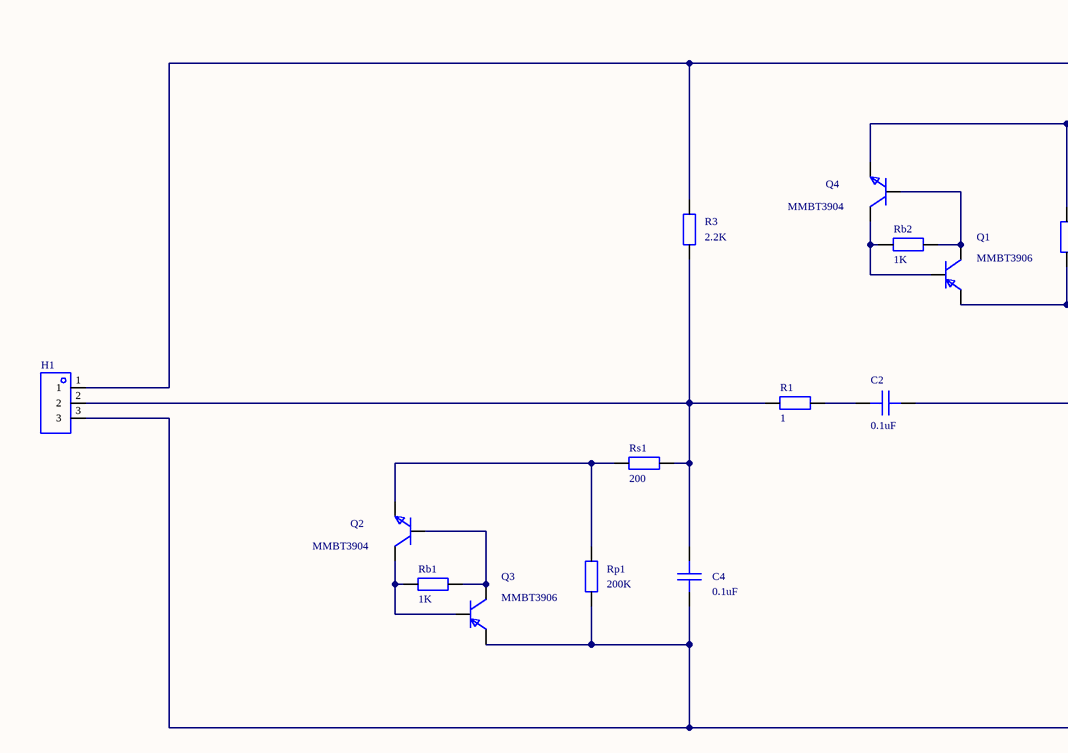
[diagram p0: MISC51432-3.schdoc, column 1 of 4]
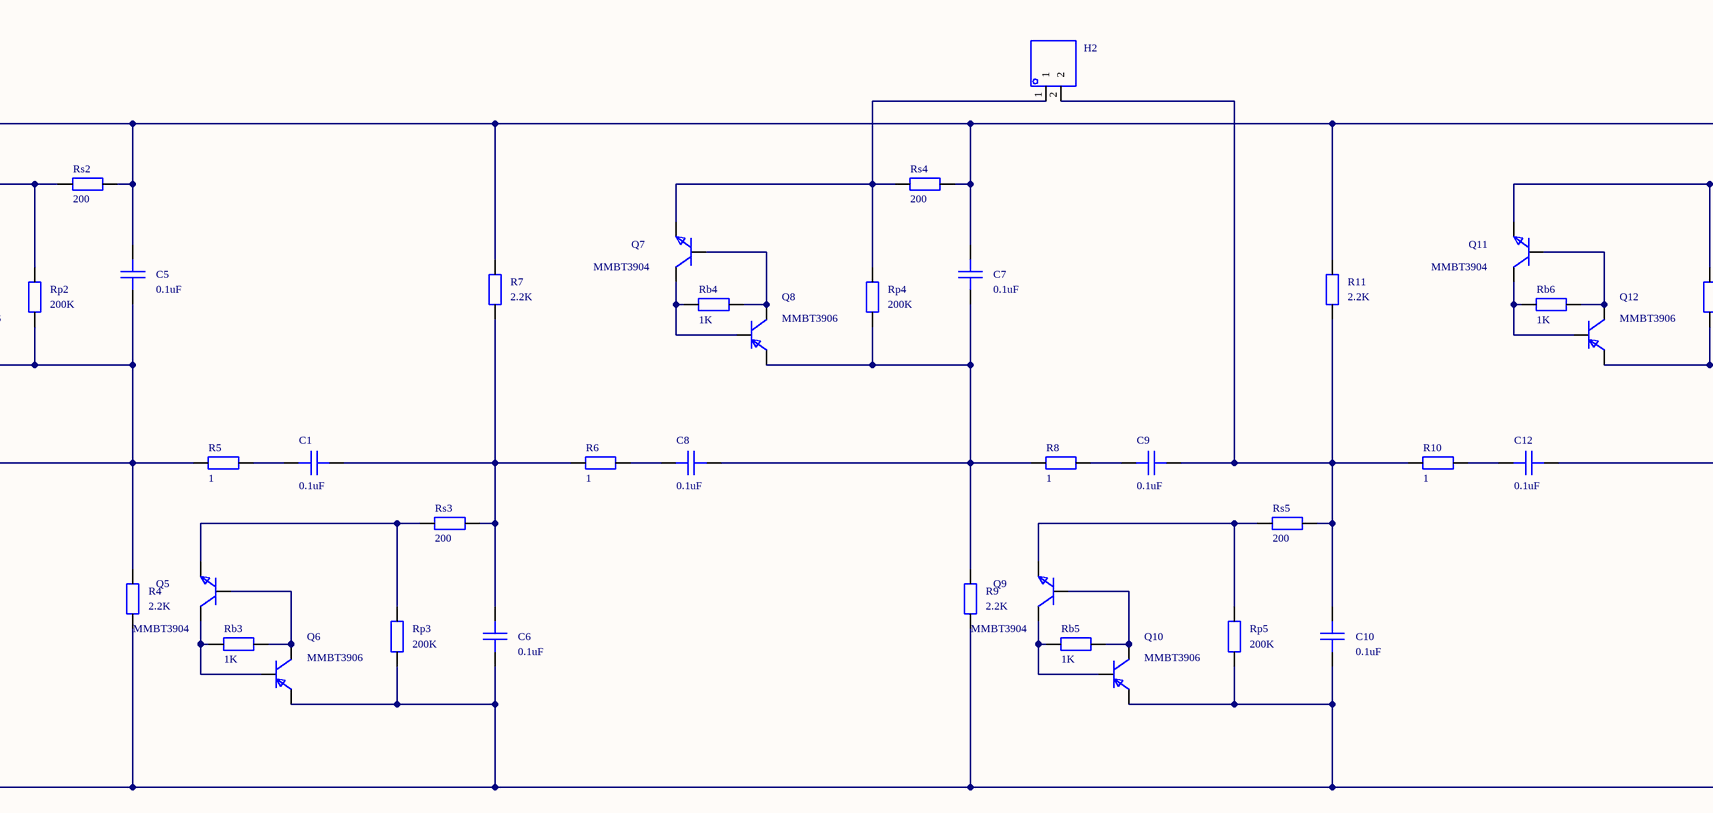
[diagram p1: MISC51432-3.schdoc, column 2 of 4]
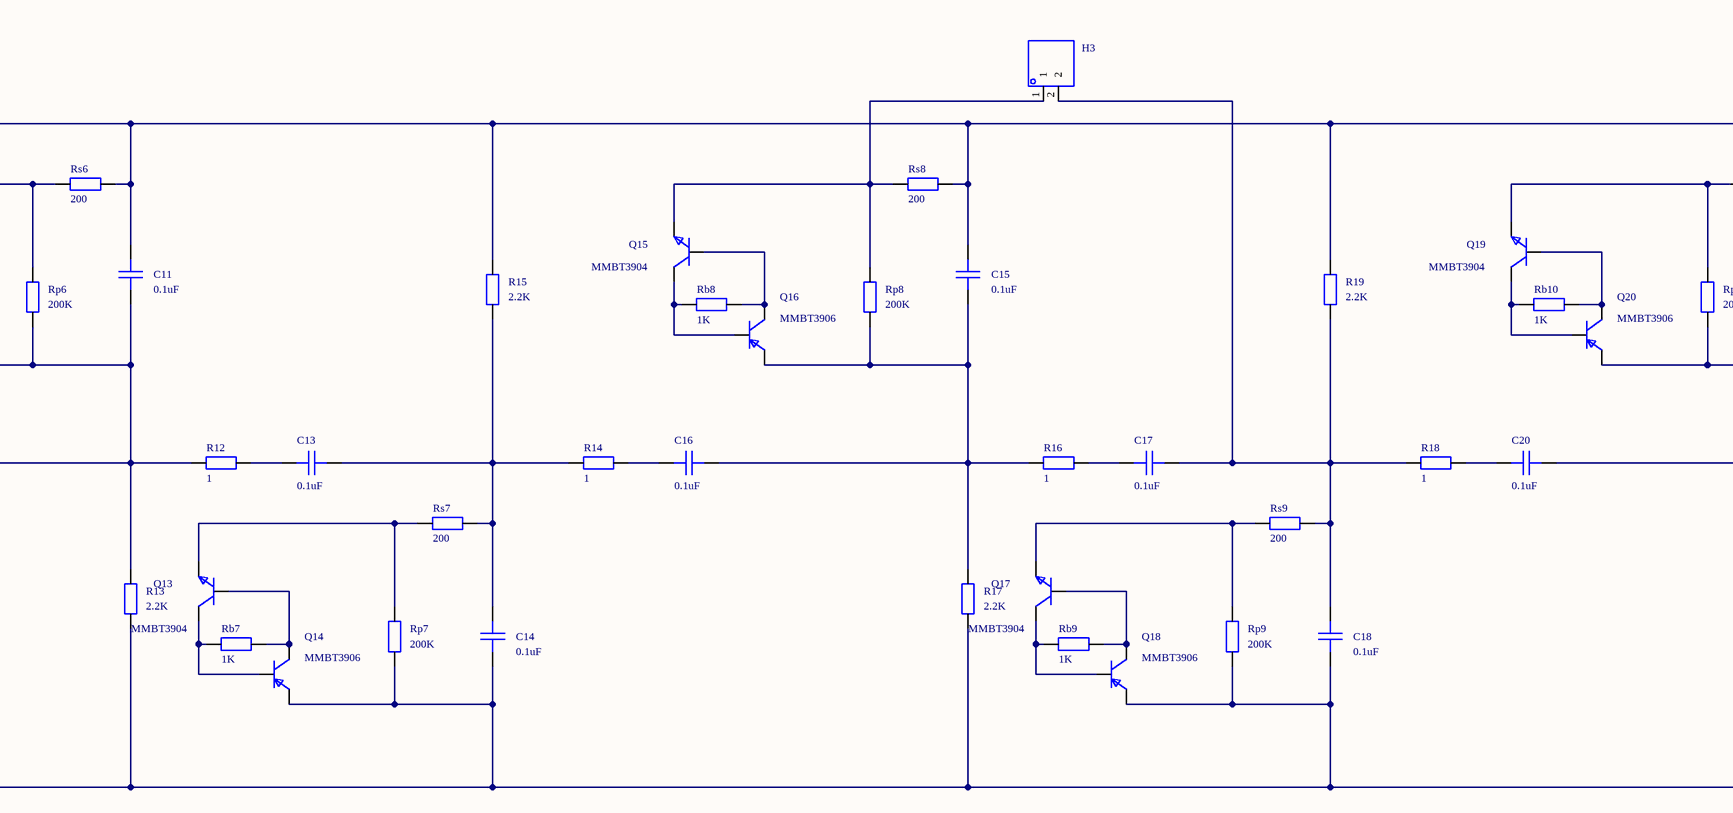
[diagram p2: MISC51432-3.schdoc, column 3 of 4]
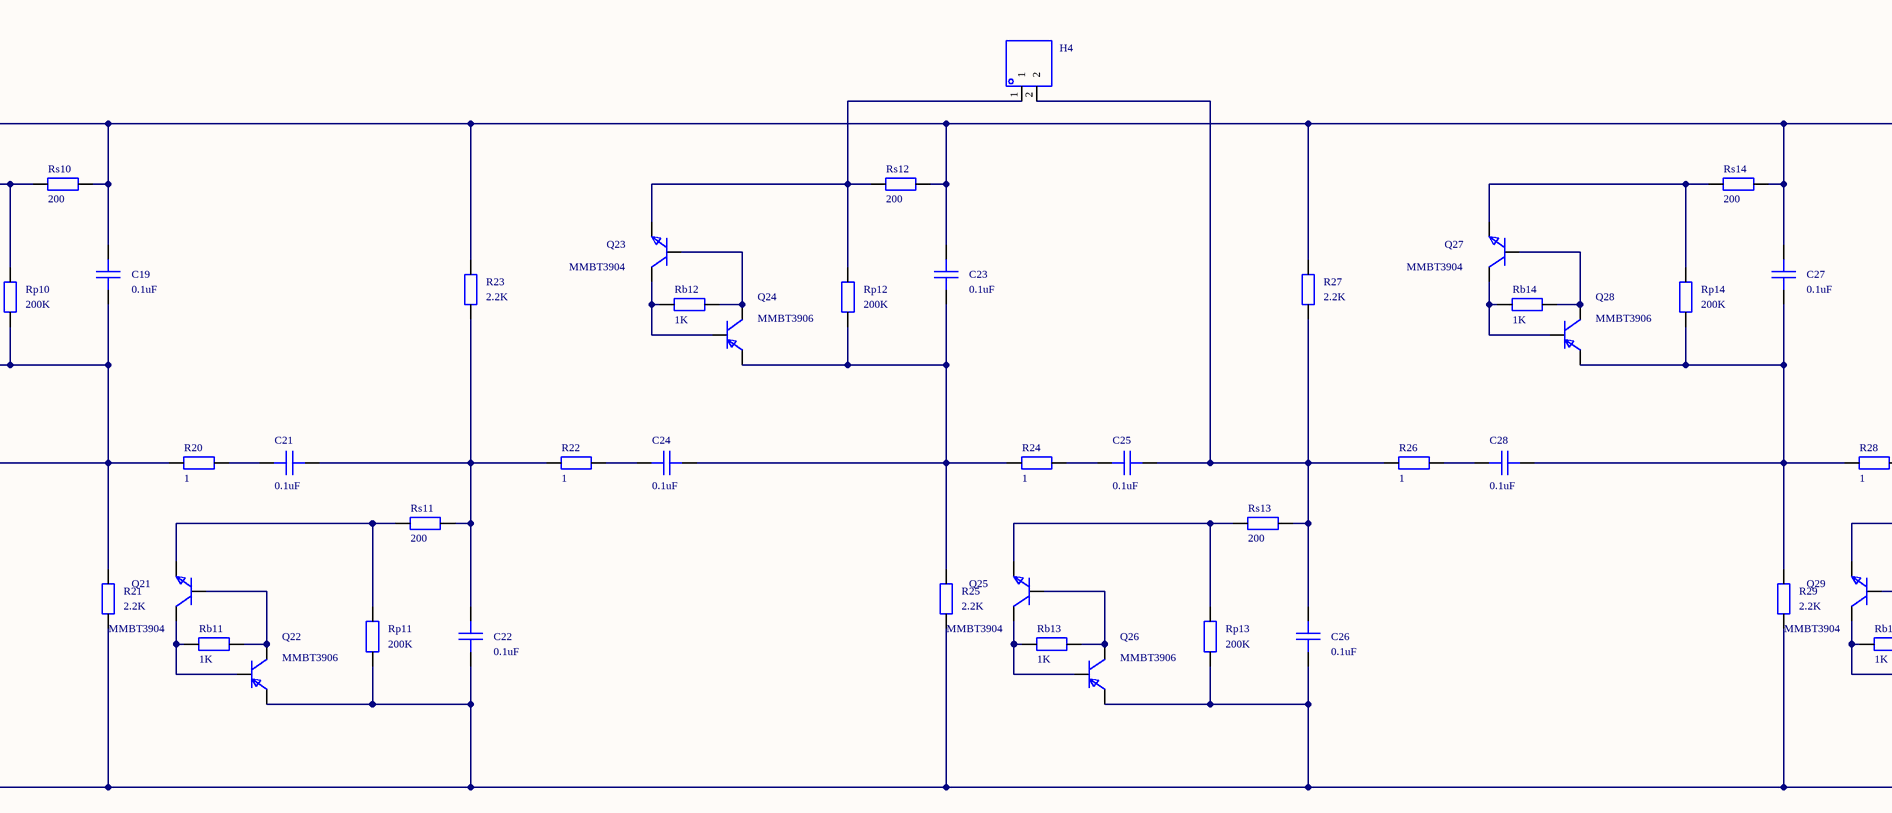
[diagram p3: MISC51432-3.schdoc, column 4 of 4]
# Altium project MISC51432-2.PrjPcb
1 sheet, 257 parts. Net scope: global (net labels, ports and power ports of the same name join across sheets).
Board file: MISC51432.pcbdoc

## Sheet MISC51432-3.schdoc
size 297 x 209 mm; Version: V1.0; @Project Name: MISC51432; @Page Count: 1; @Update Date: 2025-01-08; @Create Date: 2025-01-08; @Schematic Name: MISC51432; @Page No: 1; @Board Name: MISC51432; @Create Time: 14:24:57; @Update Time: 14:24:57

### Parts
C1  0.1uF  [C0402]
C2  0.1uF  [C0402]
C4  0.1uF  [C0402]
C5  0.1uF  [C0402]
C6  0.1uF  [C0402]
C7  0.1uF  [C0402]
C8  0.1uF  [C0402]
C9  0.1uF  [C0402]
C10  0.1uF  [C0402]
C11  0.1uF  [C0402]
C12  0.1uF  [C0402]
C13  0.1uF  [C0402]
C14  0.1uF  [C0402]
C15  0.1uF  [C0402]
C16  0.1uF  [C0402]
C17  0.1uF  [C0402]
C18  0.1uF  [C0402]
C19  0.1uF  [C0402]
C20  0.1uF  [C0402]
C21  0.1uF  [C0402]
C22  0.1uF  [C0402]
C23  0.1uF  [C0402]
C24  0.1uF  [C0402]
C25  0.1uF  [C0402]
C26  0.1uF  [C0402]
C27  0.1uF  [C0402]
C28  0.1uF  [C0402]
C29  0.1uF  [C0402]
C30  0.1uF  [C0402]
C31  0.1uF  [C0402]
C32  0.1uF  [C0402]
C33  0.1uF  [C0402]
C34  0.1uF  [C0402]
C35  0.1uF  [C0402]
C36  0.1uF  [C0402]
C37  0.1uF  [C0402]
C38  0.1uF  [C0402]
C39  0.1uF  [C0402]
C40  0.1uF  [C0402]
C41  0.1uF  [C0402]
C42  0.1uF  [C0402]
C43  0.1uF  [C0402]
C44  0.1uF  [C0402]
C45  0.1uF  [C0402]
C46  0.1uF  [C0402]
C47  0.1uF  [C0402]
C48  0.1uF  [C0402]
C49  0.1uF  [C0402]
C50  0.1uF  [C0402]
C51  0.1uF  [C0402]
C52  0.1uF  [C0402]
C53  0.1uF  [C0402]
C54  0.1uF  [C0402]
C55  0.1uF  [C0402]
C56  0.1uF  [C0402]
H1  (no value)  [HDR-TH_3P-P2.54-V-M]
H2  (no value)  [HDR-TH_2P-P2.54-V-M-1]
H3  (no value)  [HDR-TH_2P-P2.54-V-M-1]
H4  (no value)  [HDR-TH_2P-P2.54-V-M-1]
H5  (no value)  [HDR-TH_2P-P2.54-V-M-1]
H6  (no value)  [HDR-TH_2P-P2.54-V-M-1]
H7  (no value)  [HDR-TH_2P-P2.54-V-M-1]
Q1  MMBT3906  [SOT-23-3_L2.9-W1.3-P1.90-LS2.4-BR]
Q2  MMBT3904  [SOT-23-3_L2.9-W1.3-P1.90-LS2.4-BR]
Q3  MMBT3906  [SOT-23-3_L2.9-W1.3-P1.90-LS2.4-BR]
Q4  MMBT3904  [SOT-23-3_L2.9-W1.3-P1.90-LS2.4-BR]
Q5  MMBT3904  [SOT-23-3_L2.9-W1.3-P1.90-LS2.4-BR]
Q6  MMBT3906  [SOT-23-3_L2.9-W1.3-P1.90-LS2.4-BR]
Q7  MMBT3904  [SOT-23-3_L2.9-W1.3-P1.90-LS2.4-BR]
Q8  MMBT3906  [SOT-23-3_L2.9-W1.3-P1.90-LS2.4-BR]
Q9  MMBT3904  [SOT-23-3_L2.9-W1.3-P1.90-LS2.4-BR]
Q10  MMBT3906  [SOT-23-3_L2.9-W1.3-P1.90-LS2.4-BR]
Q11  MMBT3904  [SOT-23-3_L2.9-W1.3-P1.90-LS2.4-BR]
Q12  MMBT3906  [SOT-23-3_L2.9-W1.3-P1.90-LS2.4-BR]
Q13  MMBT3904  [SOT-23-3_L2.9-W1.3-P1.90-LS2.4-BR]
Q14  MMBT3906  [SOT-23-3_L2.9-W1.3-P1.90-LS2.4-BR]
Q15  MMBT3904  [SOT-23-3_L2.9-W1.3-P1.90-LS2.4-BR]
Q16  MMBT3906  [SOT-23-3_L2.9-W1.3-P1.90-LS2.4-BR]
Q17  MMBT3904  [SOT-23-3_L2.9-W1.3-P1.90-LS2.4-BR]
Q18  MMBT3906  [SOT-23-3_L2.9-W1.3-P1.90-LS2.4-BR]
Q19  MMBT3904  [SOT-23-3_L2.9-W1.3-P1.90-LS2.4-BR]
Q20  MMBT3906  [SOT-23-3_L2.9-W1.3-P1.90-LS2.4-BR]
Q21  MMBT3904  [SOT-23-3_L2.9-W1.3-P1.90-LS2.4-BR]
Q22  MMBT3906  [SOT-23-3_L2.9-W1.3-P1.90-LS2.4-BR]
Q23  MMBT3904  [SOT-23-3_L2.9-W1.3-P1.90-LS2.4-BR]
Q24  MMBT3906  [SOT-23-3_L2.9-W1.3-P1.90-LS2.4-BR]
Q25  MMBT3904  [SOT-23-3_L2.9-W1.3-P1.90-LS2.4-BR]
Q26  MMBT3906  [SOT-23-3_L2.9-W1.3-P1.90-LS2.4-BR]
Q27  MMBT3904  [SOT-23-3_L2.9-W1.3-P1.90-LS2.4-BR]
Q28  MMBT3906  [SOT-23-3_L2.9-W1.3-P1.90-LS2.4-BR]
Q29  MMBT3904  [SOT-23-3_L2.9-W1.3-P1.90-LS2.4-BR]
Q30  MMBT3906  [SOT-23-3_L2.9-W1.3-P1.90-LS2.4-BR]
Q31  MMBT3904  [SOT-23-3_L2.9-W1.3-P1.90-LS2.4-BR]
Q32  MMBT3906  [SOT-23-3_L2.9-W1.3-P1.90-LS2.4-BR]
Q33  MMBT3904  [SOT-23-3_L2.9-W1.3-P1.90-LS2.4-BR]
Q34  MMBT3906  [SOT-23-3_L2.9-W1.3-P1.90-LS2.4-BR]
Q35  MMBT3904  [SOT-23-3_L2.9-W1.3-P1.90-LS2.4-BR]
Q36  MMBT3906  [SOT-23-3_L2.9-W1.3-P1.90-LS2.4-BR]
Q37  MMBT3904  [SOT-23-3_L2.9-W1.3-P1.90-LS2.4-BR]
Q38  MMBT3906  [SOT-23-3_L2.9-W1.3-P1.90-LS2.4-BR]
Q39  MMBT3904  [SOT-23-3_L2.9-W1.3-P1.90-LS2.4-BR]
Q40  MMBT3906  [SOT-23-3_L2.9-W1.3-P1.90-LS2.4-BR]
Q41  MMBT3904  [SOT-23-3_L2.9-W1.3-P1.90-LS2.4-BR]
Q42  MMBT3906  [SOT-23-3_L2.9-W1.3-P1.90-LS2.4-BR]
Q43  MMBT3904  [SOT-23-3_L2.9-W1.3-P1.90-LS2.4-BR]
Q44  MMBT3906  [SOT-23-3_L2.9-W1.3-P1.90-LS2.4-BR]
Q45  MMBT3904  [SOT-23-3_L2.9-W1.3-P1.90-LS2.4-BR]
Q46  MMBT3906  [SOT-23-3_L2.9-W1.3-P1.90-LS2.4-BR]
Q47  MMBT3904  [SOT-23-3_L2.9-W1.3-P1.90-LS2.4-BR]
Q48  MMBT3906  [SOT-23-3_L2.9-W1.3-P1.90-LS2.4-BR]
Q49  MMBT3904  [SOT-23-3_L2.9-W1.3-P1.90-LS2.4-BR]
Q50  MMBT3906  [SOT-23-3_L2.9-W1.3-P1.90-LS2.4-BR]
Q51  MMBT3904  [SOT-23-3_L2.9-W1.3-P1.90-LS2.4-BR]
Q52  MMBT3906  [SOT-23-3_L2.9-W1.3-P1.90-LS2.4-BR]
Q53  MMBT3904  [SOT-23-3_L2.9-W1.3-P1.90-LS2.4-BR]
Q54  MMBT3906  [SOT-23-3_L2.9-W1.3-P1.90-LS2.4-BR]
Q55  MMBT3904  [SOT-23-3_L2.9-W1.3-P1.90-LS2.4-BR]
Q56  MMBT3906  [SOT-23-3_L2.9-W1.3-P1.90-LS2.4-BR]
R1  1  [R0402]
R3  2.2K  [R0402]
R4  2.2K  [R0402]
R5  1  [R0402]
R6  1  [R0402]
R7  2.2K  [R0402]
R8  1  [R0402]
R9  2.2K  [R0402]
R10  1  [R0402]
R11  2.2K  [R0402]
R12  1  [R0402]
R13  2.2K  [R0402]
R14  1  [R0402]
R15  2.2K  [R0402]
R16  1  [R0402]
R17  2.2K  [R0402]
R18  1  [R0402]
R19  2.2K  [R0402]
R20  1  [R0402]
R21  2.2K  [R0402]
R22  1  [R0402]
R23  2.2K  [R0402]
R24  1  [R0402]
R25  2.2K  [R0402]
R26  1  [R0402]
R27  2.2K  [R0402]
R28  1  [R0402]
R29  2.2K  [R0402]
R30  1  [R0402]
R31  2.2K  [R0402]
R32  1  [R0402]
R33  2.2K  [R0402]
R34  1  [R0402]
R35  2.2K  [R0402]
R36  1  [R0402]
R37  2.2K  [R0402]
R38  1  [R0402]
R39  2.2K  [R0402]
R40  1  [R0402]
R41  2.2K  [R0402]
R42  1  [R0402]
R43  2.2K  [R0402]
R44  1  [R0402]
R45  2.2K  [R0402]
R46  1  [R0402]
R47  2.2K  [R0402]
R48  1  [R0402]
R49  2.2K  [R0402]
R50  1  [R0402]
R51  2.2K  [R0402]
R52  1  [R0402]
R53  2.2K  [R0402]
R54  1  [R0402]
R55  2.2K  [R0402]
R56  2.2K  [R0402]
Rb1  1K  [R0402]
Rb2  1K  [R0402]
Rb3  1K  [R0402]
Rb4  1K  [R0402]
Rb5  1K  [R0402]
Rb6  1K  [R0402]
Rb7  1K  [R0402]
Rb8  1K  [R0402]
Rb9  1K  [R0402]
Rb10  1K  [R0402]
Rb11  1K  [R0402]
Rb12  1K  [R0402]
Rb13  1K  [R0402]
Rb14  1K  [R0402]
Rb15  1K  [R0402]
Rb16  1K  [R0402]
Rb17  1K  [R0402]
Rb18  1K  [R0402]
Rb19  1K  [R0402]
Rb20  1K  [R0402]
Rb21  1K  [R0402]
Rb22  1K  [R0402]
Rb23  1K  [R0402]
Rb24  1K  [R0402]
Rb25  1K  [R0402]
Rb26  1K  [R0402]
Rb27  1K  [R0402]
Rb28  1K  [R0402]
Rp1  200K  [R0402]
Rp2  200K  [R0402]
Rp3  200K  [R0402]
Rp4  200K  [R0402]
Rp5  200K  [R0402]
Rp6  200K  [R0402]
Rp7  200K  [R0402]
Rp8  200K  [R0402]
Rp9  200K  [R0402]
Rp10  200K  [R0402]
Rp11  200K  [R0402]
Rp12  200K  [R0402]
Rp13  200K  [R0402]
Rp14  200K  [R0402]
Rp15  200K  [R0402]
Rp16  200K  [R0402]
Rp17  200K  [R0402]
Rp18  200K  [R0402]
Rp19  200K  [R0402]
Rp20  200K  [R0402]
Rp21  200K  [R0402]
Rp22  200K  [R0402]
Rp23  200K  [R0402]
Rp24  200K  [R0402]
Rp25  200K  [R0402]
Rp26  200K  [R0402]
Rp27  200K  [R0402]
Rp28  200K  [R0402]
Rs1  200  [R0402]
Rs2  200  [R0402]
Rs3  200  [R0402]
Rs4  200  [R0402]
Rs5  200  [R0402]
Rs6  200  [R0402]
Rs7  200  [R0402]
Rs8  200  [R0402]
Rs9  200  [R0402]
Rs10  200  [R0402]
Rs11  200  [R0402]
Rs12  200  [R0402]
Rs13  200  [R0402]
Rs14  200  [R0402]
Rs15  200  [R0402]
Rs16  200  [R0402]
Rs17  200  [R0402]
Rs18  200  [R0402]
Rs19  200  [R0402]
Rs20  200  [R0402]
Rs21  200  [R0402]
Rs22  200  [R0402]
Rs23  200  [R0402]
Rs24  200  [R0402]
Rs25  200  [R0402]
Rs26  200  [R0402]
Rs27  200  [R0402]
Rs28  200  [R0402]

### Nets
NetC1_1: C1.1 C6.2 R6.2 R7.1 Rs3.2
NetC1_2: C1.2 R5.1
NetC2_1: C2.1 C5.1 Q1.2(E) R4.2 R5.2 Rp2.1
NetC2_2: C2.2 R1.1
NetC4_1: C4.1 C6.1 C10.1 C14.1 C18.1 C22.1 C26.1 C30.1 C34.1 C38.1 C42.1 C46.1 C50.1 C54.1 H1.3 Q3.2(E) Q6.2(E) Q10.2(E) Q14.2(E) Q18.2(E) Q22.2(E) Q26.2(E) Q30.2(E) Q34.2(E) Q38.2(E) Q42.2(E) Q46.2(E) Q50.2(E) Q54.2(E) R4.1 R9.1 R13.1 R17.1 R21.1 R25.1 R29.1 R33.1 R37.1 R41.1 R45.1 R49.1 R53.1 R56.1 Rp1.1 Rp3.1 Rp5.1 Rp7.1 Rp9.1 Rp11.1 Rp13.1 Rp15.1 Rp17.1 Rp19.1 Rp21.1 Rp23.1 Rp25.1 Rp27.1
NetC4_2: C4.2 H1.2 R1.2 R3.1 Rs1.2
NetC5_2: C5.2 C7.2 C11.2 C15.2 C19.2 C23.2 C27.2 C31.2 C35.2 C39.2 C43.2 C47.2 C51.2 C55.2 H1.1 R3.2 R7.2 R11.2 R15.2 R19.2 R23.2 R27.2 R31.2 R35.2 R39.2 R43.2 R47.2 R51.2 R55.2 Rs2.2 Rs4.2 Rs6.2 Rs8.2 Rs10.2 Rs12.2 Rs14.2 Rs16.2 Rs18.2 Rs20.2 Rs22.2 Rs24.2 Rs26.2 Rs28.2
NetC7_1: C7.1 C8.1 Q8.2(E) R8.2 R9.2 Rp4.1
NetC8_2: C8.2 R6.1
NetC9_1: C9.1 C10.2 H2.2 R10.2 R11.1 Rs5.2
NetC9_2: C9.2 R8.1
NetC11_1: C11.1 C12.1 Q12.2(E) R12.2 R13.2 Rp6.1
NetC12_2: C12.2 R10.1
NetC13_1: C13.1 C14.2 R14.2 R15.1 Rs7.2
NetC13_2: C13.2 R12.1
NetC15_1: C15.1 C16.1 Q16.2(E) R16.2 R17.2 Rp8.1
NetC16_2: C16.2 R14.1
NetC17_1: C17.1 C18.2 H3.2 R18.2 R19.1 Rs9.2
NetC17_2: C17.2 R16.1
NetC19_1: C19.1 C20.1 Q20.2(E) R20.2 R21.2 Rp10.1
NetC20_2: C20.2 R18.1
NetC21_1: C21.1 C22.2 R22.2 R23.1 Rs11.2
NetC21_2: C21.2 R20.1
NetC23_1: C23.1 C24.1 Q24.2(E) R24.2 R25.2 Rp12.1
NetC24_2: C24.2 R22.1
NetC25_1: C25.1 C26.2 H4.2 R26.2 R27.1 Rs13.2
NetC25_2: C25.2 R24.1
NetC27_1: C27.1 C28.1 Q28.2(E) R28.2 R29.2 Rp14.1
NetC28_2: C28.2 R26.1
NetC29_1: C29.1 C30.2 R30.2 R31.1 Rs15.2
NetC29_2: C29.2 R28.1
NetC31_1: C31.1 C32.1 Q32.2(E) R32.2 R33.2 Rp16.1
NetC32_2: C32.2 R30.1
NetC33_1: C33.1 C34.2 H5.2 R34.2 R35.1 Rs17.2
NetC33_2: C33.2 R32.1
NetC35_1: C35.1 C36.1 Q36.2(E) R36.2 R37.2 Rp18.1
NetC36_2: C36.2 R34.1
NetC37_1: C37.1 C38.2 R38.2 R39.1 Rs19.2
NetC37_2: C37.2 R36.1
NetC39_1: C39.1 C40.1 Q40.2(E) R40.2 R41.2 Rp20.1
NetC40_2: C40.2 R38.1
NetC41_1: C41.1 C42.2 H6.2 R42.2 R43.1 Rs21.2
NetC41_2: C41.2 R40.1
NetC43_1: C43.1 C44.1 Q44.2(E) R44.2 R45.2 Rp22.1
NetC44_2: C44.2 R42.1
NetC45_1: C45.1 C46.2 R46.2 R47.1 Rs23.2
NetC45_2: C45.2 R44.1
NetC47_1: C47.1 C48.1 Q48.2(E) R48.2 R49.2 Rp24.1
NetC48_2: C48.2 R46.1
NetC49_1: C49.1 C50.2 H7.2 R50.2 R51.1 Rs25.2
NetC49_2: C49.2 R48.1
NetC51_1: C51.1 C52.1 Q52.2(E) R52.2 R53.2 Rp26.1
NetC52_2: C52.2 R50.1
NetC53_1: C53.1 C54.2 R54.2 R55.1 Rs27.2
NetC53_2: C53.2 R52.1
NetC55_1: C55.1 C56.1 Q56.2(E) R56.2 Rp28.1
NetC56_2: C56.2 R54.1
NetH2_1: H2.1 Q7.2(E) Rp4.2 Rs4.1
NetH3_1: H3.1 Q15.2(E) Rp8.2 Rs8.1
NetH4_1: H4.1 Q23.2(E) Rp12.2 Rs12.1
NetH5_1: H5.1 Q31.2(E) Rp16.2 Rs16.1
NetH6_1: H6.1 Q39.2(E) Rp20.2 Rs20.1
NetH7_1: H7.1 Q47.2(E) Rp24.2 Rs24.1
NetQ1_1: Q1.1(B) Q4.3(C) Rb2.2
NetQ1_3: Q1.3(C) Q4.1(B) Rb2.1
NetQ2_1: Q2.1(B) Q3.3(C) Rb1.1
NetQ2_2: Q2.2(E) Rp1.2 Rs1.1
NetQ2_3: Q2.3(C) Q3.1(B) Rb1.2
NetQ4_2: Q4.2(E) Rp2.2 Rs2.1
NetQ5_1: Q5.1(B) Q6.3(C) Rb3.1
NetQ5_2: Q5.2(E) Rp3.2 Rs3.1
NetQ5_3: Q5.3(C) Q6.1(B) Rb3.2
NetQ7_1: Q7.1(B) Q8.3(C) Rb4.1
NetQ7_3: Q7.3(C) Q8.1(B) Rb4.2
NetQ9_1: Q9.1(B) Q10.3(C) Rb5.1
NetQ9_2: Q9.2(E) Rp5.2 Rs5.1
NetQ9_3: Q9.3(C) Q10.1(B) Rb5.2
NetQ11_1: Q11.1(B) Q12.3(C) Rb6.1
NetQ11_2: Q11.2(E) Rp6.2 Rs6.1
NetQ11_3: Q11.3(C) Q12.1(B) Rb6.2
NetQ13_1: Q13.1(B) Q14.3(C) Rb7.1
NetQ13_2: Q13.2(E) Rp7.2 Rs7.1
NetQ13_3: Q13.3(C) Q14.1(B) Rb7.2
NetQ15_1: Q15.1(B) Q16.3(C) Rb8.1
NetQ15_3: Q15.3(C) Q16.1(B) Rb8.2
NetQ17_1: Q17.1(B) Q18.3(C) Rb9.1
NetQ17_2: Q17.2(E) Rp9.2 Rs9.1
NetQ17_3: Q17.3(C) Q18.1(B) Rb9.2
NetQ19_1: Q19.1(B) Q20.3(C) Rb10.1
NetQ19_2: Q19.2(E) Rp10.2 Rs10.1
NetQ19_3: Q19.3(C) Q20.1(B) Rb10.2
NetQ21_1: Q21.1(B) Q22.3(C) Rb11.1
NetQ21_2: Q21.2(E) Rp11.2 Rs11.1
NetQ21_3: Q21.3(C) Q22.1(B) Rb11.2
NetQ23_1: Q23.1(B) Q24.3(C) Rb12.1
NetQ23_3: Q23.3(C) Q24.1(B) Rb12.2
NetQ25_1: Q25.1(B) Q26.3(C) Rb13.1
NetQ25_2: Q25.2(E) Rp13.2 Rs13.1
NetQ25_3: Q25.3(C) Q26.1(B) Rb13.2
NetQ27_1: Q27.1(B) Q28.3(C) Rb14.1
NetQ27_2: Q27.2(E) Rp14.2 Rs14.1
NetQ27_3: Q27.3(C) Q28.1(B) Rb14.2
NetQ29_1: Q29.1(B) Q30.3(C) Rb15.1
NetQ29_2: Q29.2(E) Rp15.2 Rs15.1
NetQ29_3: Q29.3(C) Q30.1(B) Rb15.2
NetQ31_1: Q31.1(B) Q32.3(C) Rb16.1
NetQ31_3: Q31.3(C) Q32.1(B) Rb16.2
NetQ33_1: Q33.1(B) Q34.3(C) Rb17.1
NetQ33_2: Q33.2(E) Rp17.2 Rs17.1
NetQ33_3: Q33.3(C) Q34.1(B) Rb17.2
NetQ35_1: Q35.1(B) Q36.3(C) Rb18.1
NetQ35_2: Q35.2(E) Rp18.2 Rs18.1
NetQ35_3: Q35.3(C) Q36.1(B) Rb18.2
NetQ37_1: Q37.1(B) Q38.3(C) Rb19.1
NetQ37_2: Q37.2(E) Rp19.2 Rs19.1
NetQ37_3: Q37.3(C) Q38.1(B) Rb19.2
NetQ39_1: Q39.1(B) Q40.3(C) Rb20.1
NetQ39_3: Q39.3(C) Q40.1(B) Rb20.2
NetQ41_1: Q41.1(B) Q42.3(C) Rb21.1
NetQ41_2: Q41.2(E) Rp21.2 Rs21.1
NetQ41_3: Q41.3(C) Q42.1(B) Rb21.2
NetQ43_1: Q43.1(B) Q44.3(C) Rb22.1
NetQ43_2: Q43.2(E) Rp22.2 Rs22.1
NetQ43_3: Q43.3(C) Q44.1(B) Rb22.2
NetQ45_1: Q45.1(B) Q46.3(C) Rb23.1
NetQ45_2: Q45.2(E) Rp23.2 Rs23.1
NetQ45_3: Q45.3(C) Q46.1(B) Rb23.2
NetQ47_1: Q47.1(B) Q48.3(C) Rb24.1
NetQ47_3: Q47.3(C) Q48.1(B) Rb24.2
NetQ49_1: Q49.1(B) Q50.3(C) Rb25.1
NetQ49_2: Q49.2(E) Rp25.2 Rs25.1
NetQ49_3: Q49.3(C) Q50.1(B) Rb25.2
NetQ51_1: Q51.1(B) Q52.3(C) Rb26.1
NetQ51_2: Q51.2(E) Rp26.2 Rs26.1
NetQ51_3: Q51.3(C) Q52.1(B) Rb26.2
NetQ53_1: Q53.1(B) Q54.3(C) Rb27.1
NetQ53_2: Q53.2(E) Rp27.2 Rs27.1
NetQ53_3: Q53.3(C) Q54.1(B) Rb27.2
NetQ55_1: Q55.1(B) Q56.3(C) Rb28.1
NetQ55_2: Q55.2(E) Rp28.2 Rs28.1
NetQ55_3: Q55.3(C) Q56.1(B) Rb28.2

### Notes on the sheet
- 2025-01-08
- Schematic
- Sheet
- P1
- Material code
- Reviewed
- Drawn
- Revision
- Size
- A4
- page
- 1
- Total

### Library data of the parts
C1 C2 C4-C56 = CAP_0402: ConvertToPcb: yes; SymbolName: CapAcitance; ModelId: 36a51122f27c49738f86b3bfa98863e0; ModelName: C0402_L1.0-W0.5-H0.5; ModelTransform: 39.37,19.685,0,0,0,0,0,0,0; Value: 0.1uF; Device: CAP_0402; AddInBom: yes; Supplier Footprint: 0402; FootprintName: C0402
H1 = HDR-M_2.54_1x3P: Symbol: PZ254V-11-03P_C2937625; ConvertToPcb: yes; ModelId: bb473b6d38ff42a99216a4fcdbdcc4cb; ModelName: HDR-TH_3P-P2.54-M-LI-1X3P; ModelTransform: 299.9994,100,0,0,0,0,0,0,-118.11; Device: HDR-M_2.54_1x3P; AddInBom: yes; SupplierPart: C2937625; Supplier Footprint: 插件; FootprintName: HDR-TH_3P-P2.54-V-M
H2-H7 = HDR-M_2.54_1x2P: Symbol: 210S-1*2P L=11.6MMGold-plated black; ConvertToPcb: yes; ModelId: 79b2e9f2d70a4d68a1b7098f27c6d4c5; ModelName: HDR-M-2.54_1x2; ModelTransform: 200,100,0,0,0,0,0,0,-118.11; Device: HDR-M_2.54_1x2P; AddInBom: yes; SupplierPart: C124375; Supplier Footprint: 插件; FootprintName: HDR-TH_2P-P2.54-V-M-1
Q1 Q3 Q6 Q8 Q10 Q12 Q14 Q16 Q18 Q20 Q22 Q24 Q26 Q28 Q30 Q32 Q34 Q36 Q38 Q40 Q42 Q44 Q46 Q48 Q50 Q52 Q54 Q56 = MMBT3906-13-01-F: Transistor type:-;Collector current(Ic):-;Collector-emitter breakdown voltage(Vceo):-;Power(Pd):-;; Manufacturer: DIODES(美台); AddInBom: yes; ModelId: c62791f0466c4ae2a892c056b845b0ca; ModelName: SOT-23-3P_L2.9-W1.3-H1.0-LS2.4-P0.95; ModelTransform: 98.425,114.173,0,180,0,0,0.0005,-0.0005,0; Symbol: MMBT3906-13-01-F; Manufacturer Part: MMBT3906; Device: MMBT3906-13-01-F; LCSC Part Name: MMBT3906-13-01-F; SupplierPart: C526675; Supplier Footprint: SOT-23-3; JLCPCB Part Class: Extended library; Supplier: LCSC; ConvertToPcb: yes; FootprintName: SOT-23-3_L2.9-W1.3-P1.90-LS2.4-BR; Transistor Type: -; Collector Current (Ic): -; Collector-Emitter Breakdown Voltage (Vceo): -; Power Dissipation (Pd): -; Transition Frequency (fT): -; Collector Cut-Off Current (Icbo): -; Collector-Emitter Saturation Voltage (VCE(sat)@Ic,Ib): -
Q2 Q4 Q5 Q7 Q9 Q11 Q13 Q15 Q17 Q19 Q21 Q23 Q25 Q27 Q29 Q31 Q33 Q35 Q37 Q39 Q41 Q43 Q45 Q47 Q49 Q51 Q53 Q55 = MMBT3904(RANGE:100-300): 晶体管类型:NPN;集电极电流(Ic):200mA;集射极击穿电压(Vceo):40V;功率(Pd):200mW;直流电流增益(hFE@Ic,Vce):100@10mA,1V;; Manufacturer: CJ(江苏长电/长晶); AddInBom: yes; ModelId: c62791f0466c4ae2a892c056b845b0ca; ModelName: SOT-23-3P_L2.9-W1.3-H1.0-LS2.4-P0.95; ModelTransform: 98.425,114.173,0,180,0,0,0.0005,-0.0005,0; Transistor Type: NPN; Collector Current (Ic): 200mA; Collector-Emitter Breakdown Voltage (Vceo): 40V; Power Dissipation (Pd): 200mW; Transition Frequency (fT): 300MHz; Collector Cut-Off Current (Icbo): 100nA; Collector-Emitter Saturation Voltage (VCE(sat)@Ic,Ib): 300mV@50mA,5mA; Symbol: MMBT3904; Manufacturer Part: MMBT3904; Device: MMBT3904(RANGE:100-300); LCSC Part Name: NPN 电流:200mA 耐压:40V hfe=100~300; SupplierPart: C20526; Supplier Footprint: SOT-23; Datasheet: https://atta.szlcsc.com/upload/public/pdf/source/20220704/70F575FB75061E03F919270A6BB8BA7F.pdf; Supplier: LCSC; ConvertToPcb: yes; FootprintName: SOT-23-3_L2.9-W1.3-P1.90-LS2.4-BR; DC Current Gain (hFE@Ic,Vce): 100@10mA,1V; Operating Temperature: -
R1 R3-R56 Rb1-Rb28 Rp1-Rp28 Rs1-Rs28 = Res_0402: Symbol: Resistor; ConvertToPcb: yes; ModelId: 671aefced39d4c318694bba8bd8efd39; ModelName: R0402_L1.0-W0.5-H0.5; ModelTransform: 39.37,19.685,0,0,0,0,0,0.0005,0; Device: Res_0402; AddInBom: yes; Supplier Footprint: 0402; FootprintName: R0402
  R1 R5 R6 R8 R10 R12 R14 R16 R18 R20 R22 R24 R26 R28 R30 R32 R34 R36 R38 R40 R42 R44 R46 R48 R50 R52 R54: Value: 1
  R3 R4 R7 R9 R11 R13 R15 R17 R19 R21 R23 R25 R27 R29 R31 R33 R35 R37 R39 R41 R43 R45 R47 R49 R51 R53 R55 R56: Value: 2.2K
  Rb1-Rb28: Value: 1K
  Rp1-Rp28: Value: 200K
  Rs1-Rs28: Value: 200